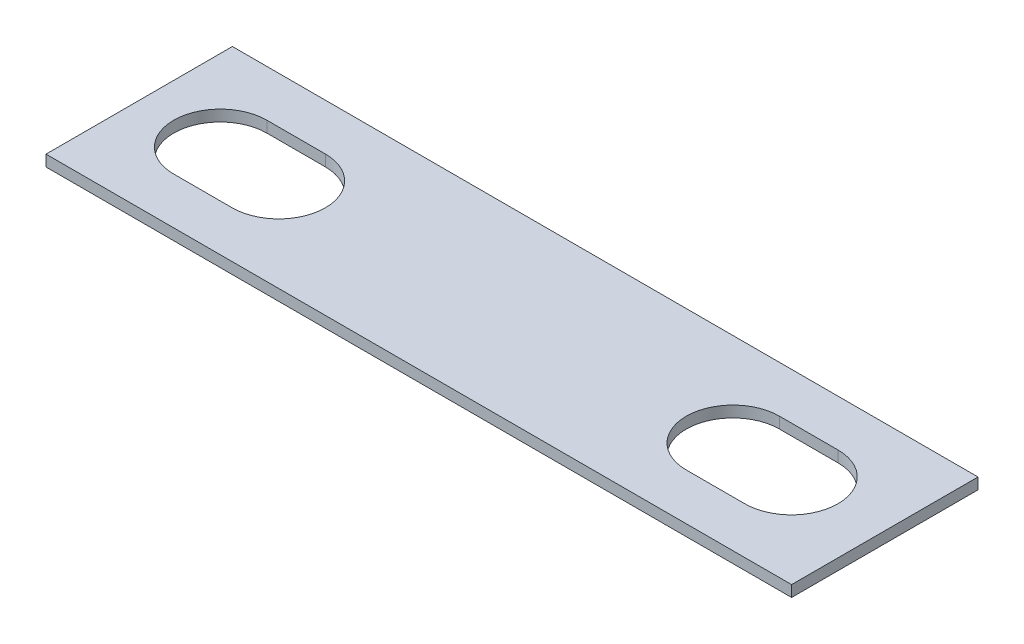
SolidWorks part; units mm, degrees
ref_plane "Front Plane" through (0, 0, 0) normal (0, 0, 1) x (1, 0, 0)
ref_plane "Top Plane" through (0, 0, 0) normal (0, 1, 0) x (1, 0, 0)
ref_plane "Right Plane" through (0, 0, 0) normal (1, 0, 0) x (0, 0, -1)
sketch "Sketch1" plane through (0, 0, 0) normal (0, 1, 0) x (1, 0, 0)
  line L0 (101.6, 12.7) -> (-8.6359, 12.7) construction
  line L1 (0, 0) -> (101.6, 0)
  line L2 (0, 0) -> (0, 25.4)
  line L3 (0, 25.4) -> (101.6, 25.4)
  line L4 (101.6, 0) -> (101.6, 25.4)
  line L5 (11.049, 12.7) -> (19.0188, 12.7) construction
  line L6 (11.049, 19.05) -> (19.0188, 19.05)
  line L7 (11.049, 6.35) -> (19.0188, 6.35)
  line L8 (80.899, 12.7) -> (88.8688, 12.7) construction
  line L9 (80.899, 19.05) -> (88.8688, 19.05)
  line L10 (80.899, 6.35) -> (88.8688, 6.35)
  arc A0 (11.049, 19.05) -> (11.049, 6.35) centre (11.049, 12.7) ccw
  arc A1 (19.0188, 6.35) -> (19.0188, 19.05) centre (19.0188, 12.7) ccw
  arc A2 (80.899, 19.05) -> (80.899, 6.35) centre (80.899, 12.7) ccw
  arc A3 (88.8688, 6.35) -> (88.8688, 19.05) centre (88.8688, 12.7) ccw
  point P9 (15.0339, 12.7)
  point P16 (84.8839, 12.7)
  dimension "D3" = 11.049
  dimension "D1" = 101.6
  dimension "D2" = 25.4
extrude "Boss-Extrude1" add sketch "Sketch1" along normal blind 1.524
